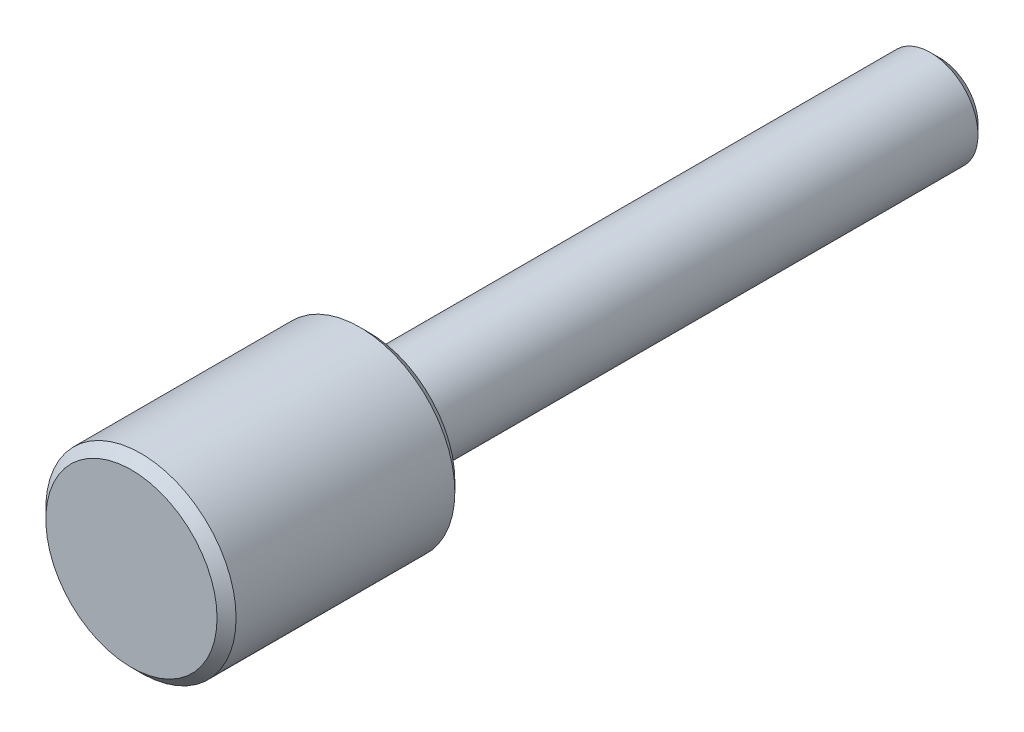
SolidWorks part; units mm, degrees
material "HSS"
ref_plane "Front Plane" through (0, 0, 0) normal (0, 0, 1) x (1, 0, 0)
ref_plane "Top Plane" through (0, 0, 0) normal (0, 1, 0) x (1, 0, 0)
ref_plane "Right Plane" through (0, 0, 0) normal (1, 0, 0) x (0, 0, -1)
sketch "Sketch1" plane through (0, 0, 0) normal (0, 0, 1) x (1, 0, 0)
  circle A0 centre (0, 0) radius 1
  dimension "D1" = 2
extrude "Boss-Extrude1" add sketch "Sketch1" along normal mid plane 17
sketch "Sketch2" plane through (0, 0, 8.5) normal (0, 0, 1) x (1, 0, 0)
  circle A0 centre (0, 0) radius 2
  dimension "D1" = 4
extrude "Boss-Extrude2" add sketch "Sketch2" against normal blind 5
chamfer "Chamfer1" distance 0.2 angle 45 3 edges at (1, 0, -8.5) (2, 0, 3.5) (2, 0, 8.5)
